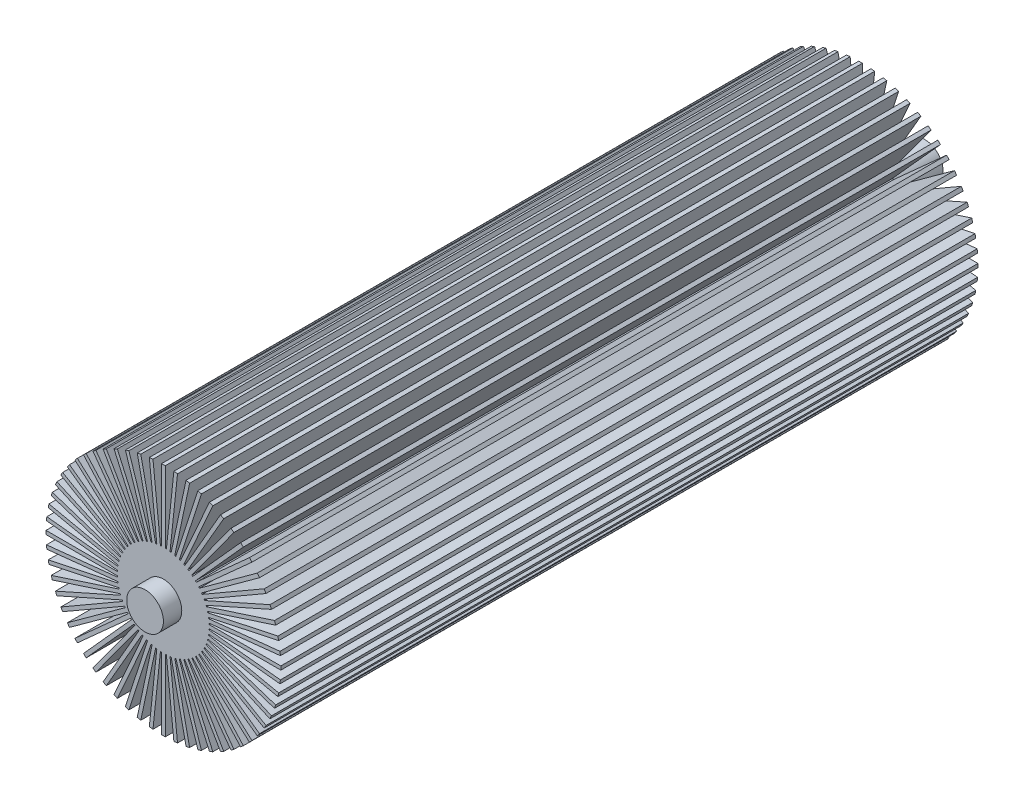
from build123d import *

# Parameters (mm, degrees)
SKETCH_1_R               = 25
EXTRUDE_1_DEPTH          = 380
SKETCH_2_R               = 10
EXTRUDE_2_DEPTH          = 10
EXTRUDE_START            = 35
SKETCH_3_R               = 10
EXTRUDE_3_DEPTH          = 35
SKETCH_4_W               = 2
SKETCH_4_H               = 40
EXTRUDE_4_DEPTH          = 380
PATTERN_CIRCULAR_1_COUNT = 60


with BuildPart() as part:
    # 草图1 → 凸台-拉伸1 (new body)
    with BuildSketch(Plane.XY):
        Circle(SKETCH_1_R)
    extrude(amount=EXTRUDE_1_DEPTH)

    # 草图2 → 凸台-拉伸2 (add)
    with BuildSketch(Plane.XY.offset(380)):
        Circle(SKETCH_2_R)
    extrude(amount=EXTRUDE_2_DEPTH)

    # 草图3 → 凸台-拉伸3 (add)
    with BuildSketch(Plane(origin=(0, 0, 0), x_dir=(-1, 0, 0), z_dir=(0, 0, -1)).offset(EXTRUDE_START)):
        with Locations(Location((0, 0, 0), (0, 0, 180))):
            Circle(SKETCH_3_R)
    extrude(amount=-EXTRUDE_3_DEPTH)

    # 草图4 → 凸台-拉伸4 (add)
    with BuildSketch(Plane(origin=(0, 0, 0), x_dir=(-1, 0, 0), z_dir=(0, 0, -1))):
        with Locations((0, 44)):
            Rectangle(SKETCH_4_W, SKETCH_4_H)
    extrude_4 = extrude(amount=-EXTRUDE_4_DEPTH)

    # 阵列(圆周)1: 凸台-拉伸4 ×60 about axis
    pattern_circular_1_axis = Axis((0, 0, 0), (0, 0, 1))
    for i in range(1, PATTERN_CIRCULAR_1_COUNT):
        add(extrude_4.rotate(pattern_circular_1_axis, i * 360 / PATTERN_CIRCULAR_1_COUNT))


solid = part.part
